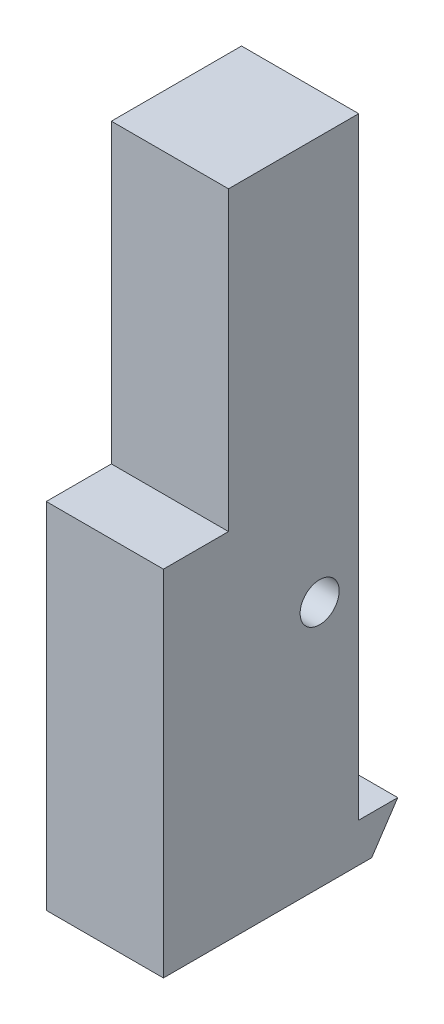
from build123d import *

# Parameters (mm, degrees)
SKETCH43_W          = 4.5
SKETCH43_H          = 25
BOSS_EXTRUDE1_DEPTH = 7.5
BOSS_EXTRUDE2_DEPTH = 4.5
SKETCH45_R          = 0.75
CUT_EXTRUDE1_DEPTH  = 16.256146302
SKETCH46_W          = 2.5
SKETCH46_H          = 11.400602873
CUT_EXTRUDE2_DEPTH  = 16.256146302


with BuildPart() as part:
    # Sketch43 → Boss-Extrude1 (new body)
    with BuildSketch(Plane.XY):
        Rectangle(SKETCH43_W, SKETCH43_H)
    extrude(amount=BOSS_EXTRUDE1_DEPTH)

    # Sketch44 → Boss-Extrude2 (add)
    with BuildSketch(Plane(origin=(2.25, 0, 0), x_dir=(0, 0, -1), z_dir=(1, 0, 0))):
        Polygon((0, -12.5), (0.5, -12.5), (1.5, -11), (0, -11), align=None)
    extrude(amount=-BOSS_EXTRUDE2_DEPTH)

    # Sketch45 → Cut-Extrude1 (cut, through all)
    with BuildSketch(Plane(origin=(2.25, 0, 0), x_dir=(0, 0, -1), z_dir=(1, 0, 0))):
        with Locations(Location((-1.5, -3, 0), (0, 0, 90))):
            Circle(SKETCH45_R)
    extrude(amount=-CUT_EXTRUDE1_DEPTH, mode=Mode.SUBTRACT)

    # Sketch46 → Cut-Extrude2 (cut, through all)
    with BuildSketch(Plane.ZY.offset(2.25)):
        with Locations((6.25, 6.799698563)):
            Rectangle(SKETCH46_W, SKETCH46_H)
    extrude(amount=-CUT_EXTRUDE2_DEPTH, mode=Mode.SUBTRACT)


solid = part.part
